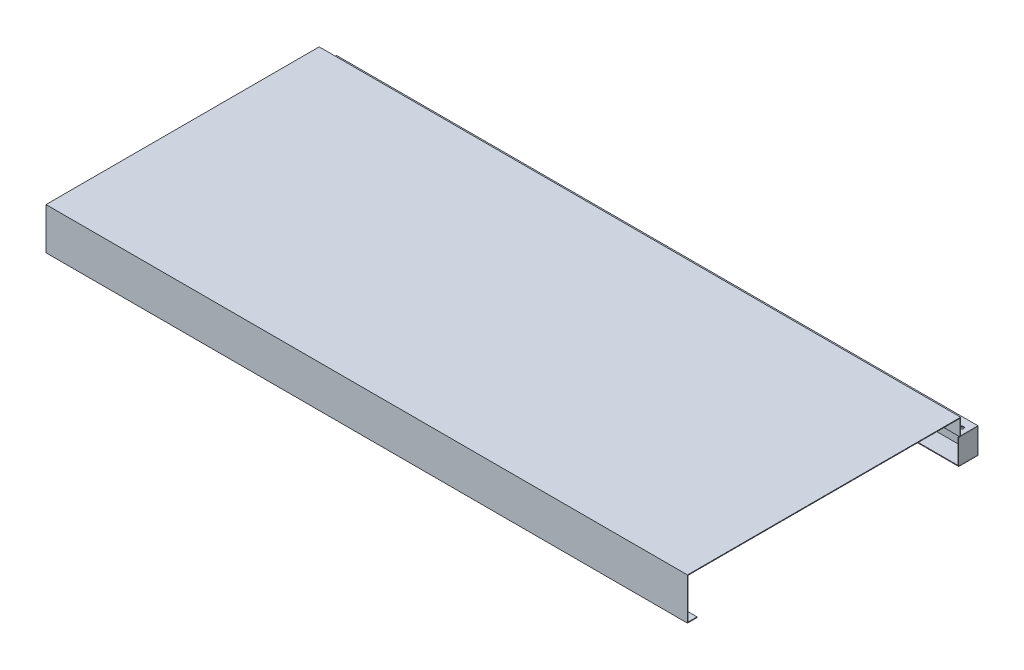
SolidWorks part; units mm, degrees
ref_plane "Front Plane" through (0, 0, 0) normal (0, 0, 1) x (1, 0, 0)
ref_plane "Top Plane" through (0, 0, 0) normal (0, 1, 0) x (1, 0, 0)
ref_plane "Right Plane" through (0, 0, 0) normal (1, 0, 0) x (0, 0, -1)
sketch "Sketch1" plane through (0, 0, 0) normal (1, 0, 0) x (0, 0, -1)
  line L0 (0, 71.9306) -> (0, -59.4209) construction
  line L1 (0, 0) -> (375, 0)
  line L2 (375, 0) -> (375, -25)
  line L3 (375, -25) -> (402, -25)
  line L4 (402, -25) -> (402, -65)
  line L5 (402, -65) -> (372, -65)
  line L6 (0, 0) -> (-50, 0)
  line L7 (-50, 0) -> (-50, -65)
  line L8 (-50, -65) -> (-35, -65)
  dimension "D1" = 40
  dimension "D2" = 25
  dimension "D3" = 30
  dimension "D4" = 65
  dimension "D5" = 15
  dimension "D6" = 425
  dimension "D7" = 452
  dimension "D8" = 50
extrude "Extrude-Thin1" add sketch "Sketch1" along normal blind 998 thin
sketch "Sketch4" plane through (0, 0, 0) normal (-1, 0, 0) x (0, 0, 1)
  line L0 (-401, -26) -> (-372, -26)
  line L1 (-372, -26) -> (-372, -64)
  line L2 (-372, -64) -> (-401, -64)
  line L3 (-401, -64) -> (-401, -26)
extrude "Extrude2" add sketch "Sketch4" against normal blind 1 separate body
sketch "Sketch5" plane through (998, 0, 0) normal (1, 0, 0) x (0, 0, -1)
  line L0 (372, -64) -> (401, -64)
  line L1 (401, -64) -> (401, -26)
  line L2 (401, -26) -> (372, -26)
  line L3 (372, -26) -> (372, -64)
  line L5 (401, -64) -> (401, -26) construction
  line L6 (401, -26) -> (401, -64) construction
  line L7 (372, -64) -> (372, -26) construction
extrude "Extrude3" add sketch "Sketch5" against normal blind 1
sketch "Sketch6" plane through (0, -25, 0) normal (0, 1, 0) x (1, 0, 0)
  line L0 (998, 402) -> (0, 402) construction
  line L1 (0, 402) -> (0, 375) construction
  line L2 (998, 402) -> (998, 375) construction
  circle A0 centre (13, 389) radius 2.75
  circle A1 centre (988, 387) radius 2.75
  dimension "D1" = 5.5
  dimension "D2" = 13
  dimension "D3" = 13
  dimension "D4" = 5.5
  dimension "D5" = 10
  dimension "D6" = 15
extrude "Cut-Extrude1" cut sketch "Sketch6" against normal blind 10
